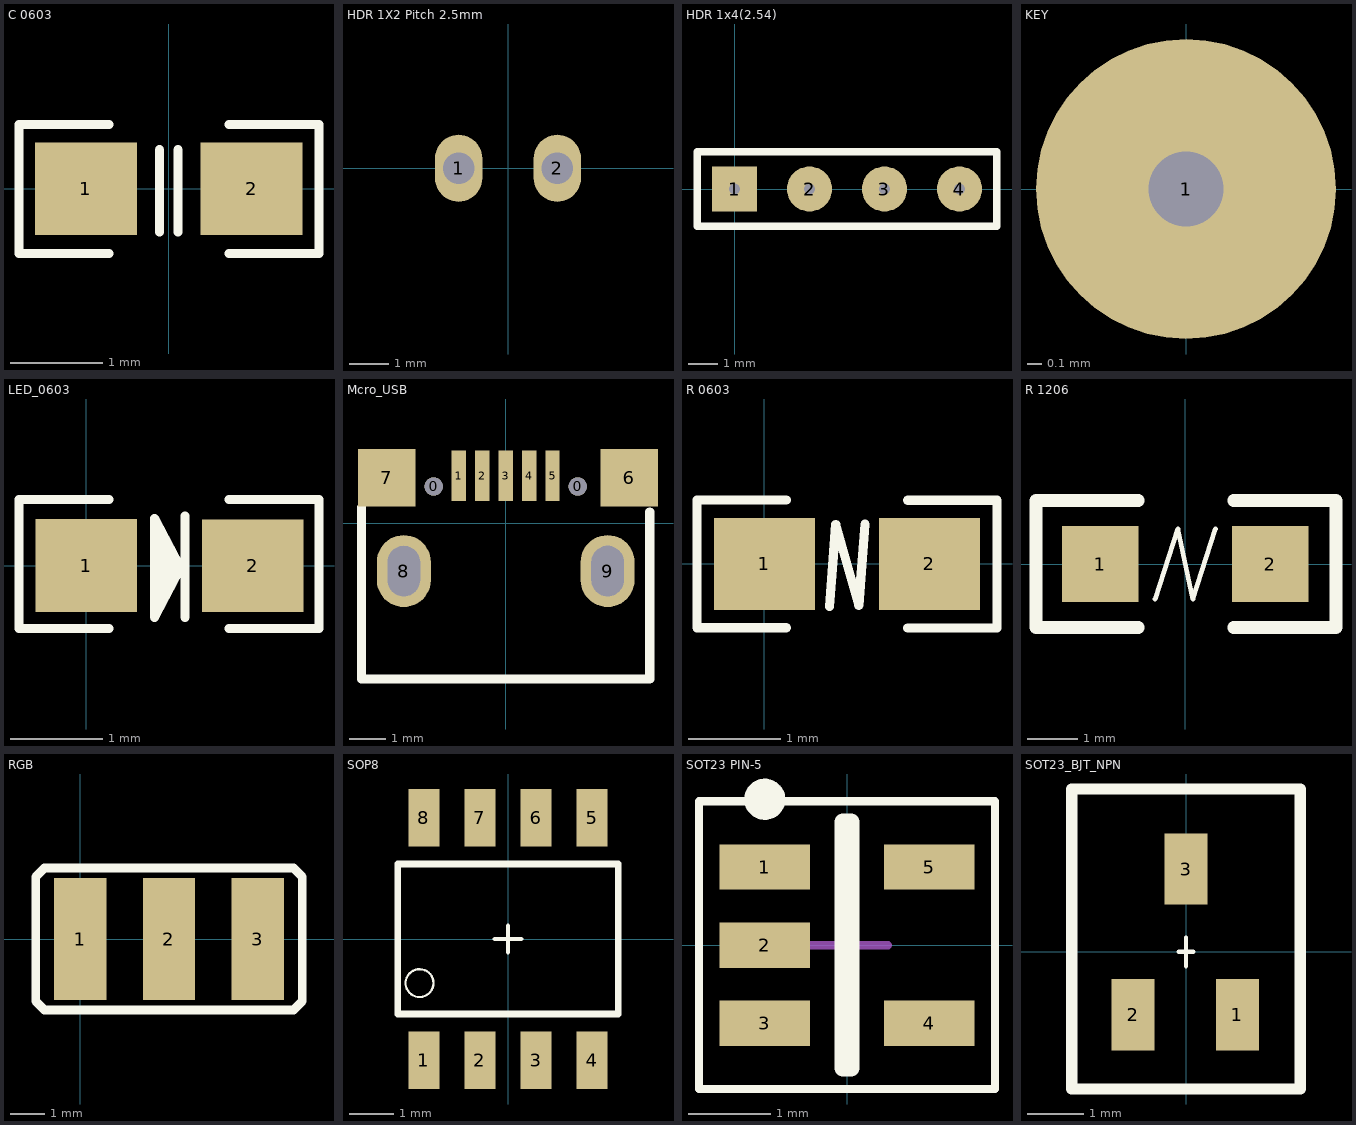
[diagram p0: the footprints below, top view; thin cyan lines are the x and y axes]
# Altium footprint library MISC64789-2.PcbLib: 12 footprints
Each footprint in its own frame and in the unit in brackets; x right, y up, seen from the top. Pads: shape width x height; smd on the part's side, far side on the other; paste and mask are expansions set on the pad; w line width, h text height; cw(c..) or ccw(c..) is an arc to the next point about the centre after c.

## C 0603 [mm] "SMD 0603 2.5x1"
pads (2):
  rect 1.1x1 smd: 1(-0.894,0) 2(0.894,0)
Top Overlay:
  lines w0.1: -0.645,-0.7 -1.617,-0.7 -1.617,0.694 -0.645,0.694 ; -0.1,-0.469 -0.1,0.42 ; 0.1,-0.469 0.1,0.42 ; 0.651,-0.701 1.623,-0.701 1.623,0.692 0.651,0.692

## HDR 1X2 Pitch 2.5mm [mm] "Header; 2 Position; Pitch 2.5"
height 1.45
pads (2):
  oval 1.2x1.7 hole 0.8: 1(-1.25,0) 2(1.25,0)
Bottom Overlay:
  lines w0.2: -1.25,2.45 -1.25,1.45 1.25,1.45 1.25,2.45 ; -3.8,-3.5 -3.8,2.45 3.8,2.45 3.8,-3.5 -3.8,-3.5

## HDR 1x4(2.54) [mil]
height 57.09
pads (4):
  rect 60x60 hole 15: 1(0,0)
  round 60 hole 15: 2(100,0) 3(200,0) 4(300,0)
Top Overlay:
  lines w10: -50,-50 350,-50 350,50 0,50 -50,50 -50,-50

## KEY [mil]
height 57.09
pads (1):
  round 80 hole 20: 1(0,0)

## LED_0603 [mm]
height 1.45
pads (2):
  rect 1.1x1 smd: 1(0,0) 2(1.798,-0.001)
Top Overlay:
  lines w0.1: 0.245,-0.68 -0.727,-0.68 -0.727,0.714 0.245,0.714 ; 0.813,-0.381 0.813,0.314 ; 0.889,-0.203 0.889,0.169 ; 0.965,-0.102 0.965,0.067 ; 1.067,-0.559 1.067,0.533 ; 1.54,-0.681 2.513,-0.681 2.513,0.712 1.54,0.712 ; 0.737,-0.559 1.016,-0.025 0.737,0.508 0.737,-0.559

## Mcro_USB [mm]
height 1.45
pads (11):
  round 0.508 hole 0.508: 0(-2,1.025) 0(2,1.025)
  rect 0.4x1.4 smd: 1(-1.3,1.325) 2(-0.65,1.325) 3(0,1.325) 4(0.65,1.325) 5(1.3,1.325)
  rect 1.6x1.6 smd: 6(3.429,1.27) 7(-3.302,1.27)
  oval 1.5x2 hole 0.9 slot 1.4 at 90 deg: 8(-2.83,-1.325) 9(2.83,-1.324)
Top Overlay:
  lines w0.254: -4,0.444 -4,-4.325 4,-4.325 4,0.318

## R 0603 [mm] "SMD 0603 2.5x1"
height 1.45
pads (2):
  rect 1.1x1 smd: 1(0,0) 2(1.798,0)
Top Overlay:
  lines w0.1: 0.239,-0.696 -0.734,-0.696 -0.734,0.697 0.239,0.697 ; 0.709,-0.462 0.778,0.429 1.028,-0.45 1.098,0.432 ; 1.564,-0.698 2.536,-0.698 2.536,0.695 1.564,0.695

## R 1206 [mil] "SMD 1206 5x1.5"
height 57.09
pads (2):
  rect 60x60 smd: 1(-66.93,0) 2(66.93,0)
Top Overlay:
  lines w3.94: -23.62,-27.56 -5.91,27.56 5.91,-27.56 23.62,27.56
  lines w10: -36.93,-50 -117.43,-50 -117.43,50 -36.93,50 ; 38.07,-50 118.57,-50 118.57,50 38.07,50

## RGB [mm]
pads (3):
  rect 1.5x3.5 smd: 1(0,0) 2(2.54,0) 3(5.08,0)
Top Overlay:
  lines w0.254: -1.27,1.524 -1.27,1.778 ; -1.27,1.778 -1.27,-1.778 -1.016,-2.032 6.096,-2.032 6.35,-1.778 6.35,1.778 6.096,2.032 -1.016,2.032 -1.27,1.778

## SOP8 [mm] "SOP8,Pitch=1.27mm,LxWxH=5.15x6.2"
height 1.5
pads (8):
  rect 0.7x1.3 smd: 1(-1.905,-2.75) 2(-0.635,-2.75) 3(0.635,-2.75) 4(1.905,-2.75) 5(1.905,2.75) 6(0.635,2.75) 7(-0.635,2.75) 8(-1.905,2.75)
Top Overlay:
  circle w0.05: c-2.005,-1 r0.316
  lines w0.1: -0.3,0 0.3,0 ; 0,-0.3 0,0.3
  lines w0.15: -2.5,-1.7 2.5,-1.7 2.5,1.7 -2.5,1.7 -2.5,-1.7

## SOT23 PIN-5 [mm]
height 1.1
pads (5):
  rect 1.1x0.55 smd: 1(-1,0.95) 2(-1,0) 3(-1,-0.95) 4(1,-0.95) 5(1,0.95)
Top Overlay:
  circle w0.25: c-1,1.775 r0.125
  lines w0.1: -1.8,-1.75 -1.8,1.75 1.8,1.75 1.8,-1.75 -1.8,-1.75
  lines w0.2: -0.05,-1.5 0.05,-1.5 0.05,1.5 -0.05,1.5 -0.05,-1.5
Mechanical 15:
  lines w0.1: -0.5,0 0.5,0 ; 0,-0.5 0,0.5

## SOT23_BJT_NPN [mil]
height 57.09
pads (3):
  rect 30x50 smd: 1(36,-44) 2(-37,-44) 3(0,58)
Top Overlay:
  lines w3: -5,0 5,0 ; 0,-10 0,10
  lines w8: -80,-96 80,-96 80,114 -80,114 -80,-96